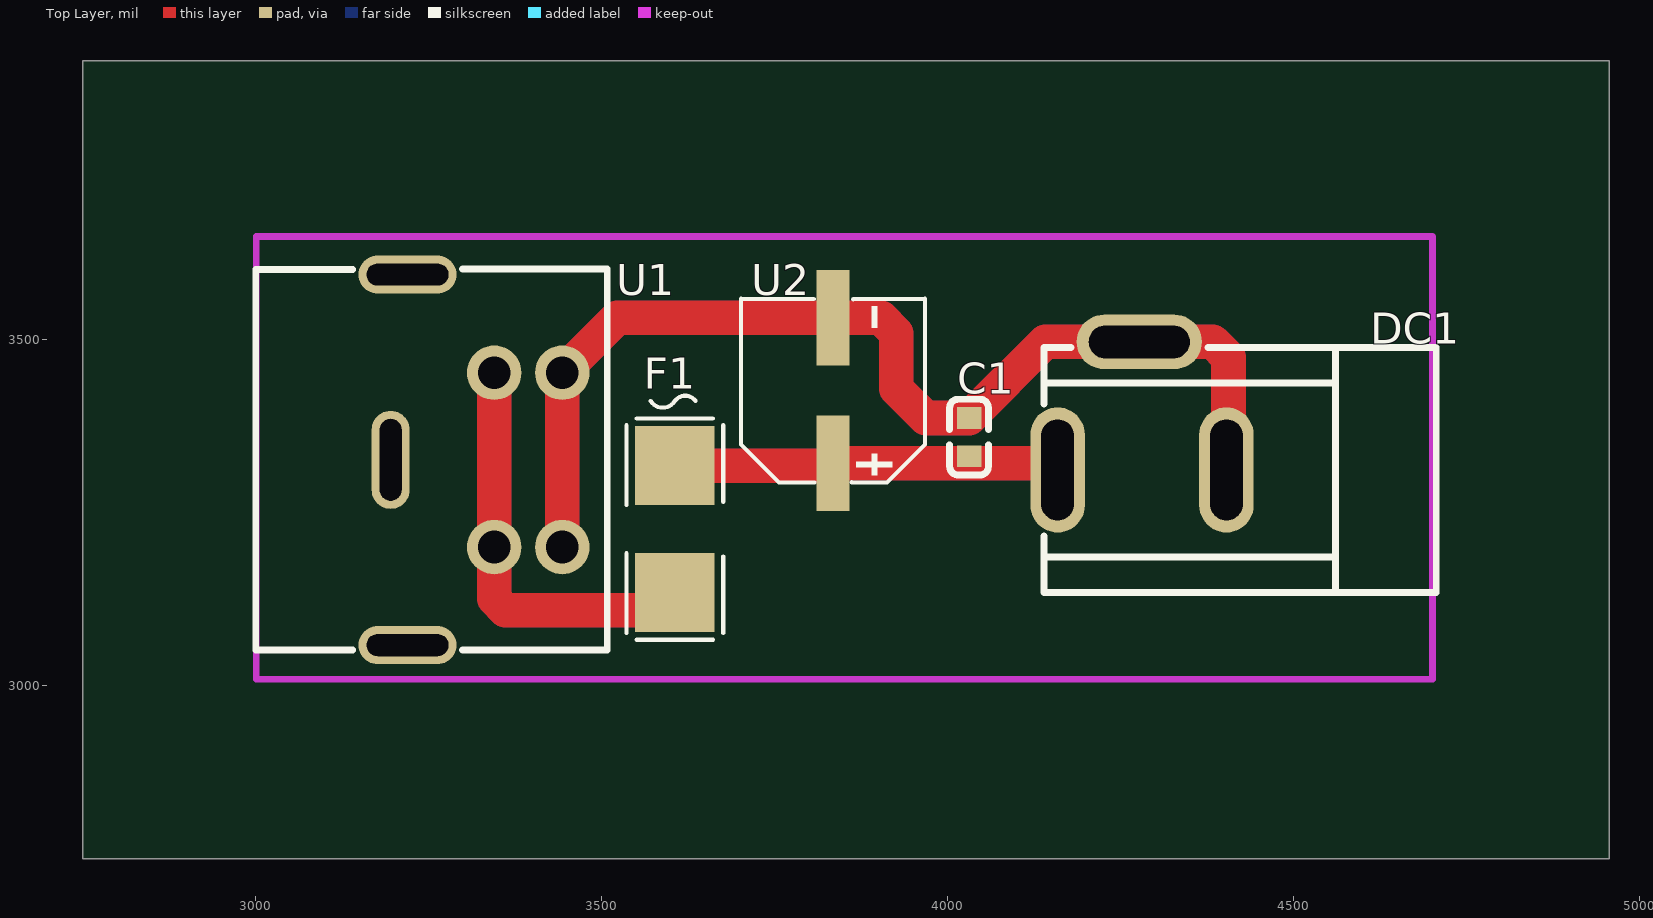
[diagram p0: Top Layer view]
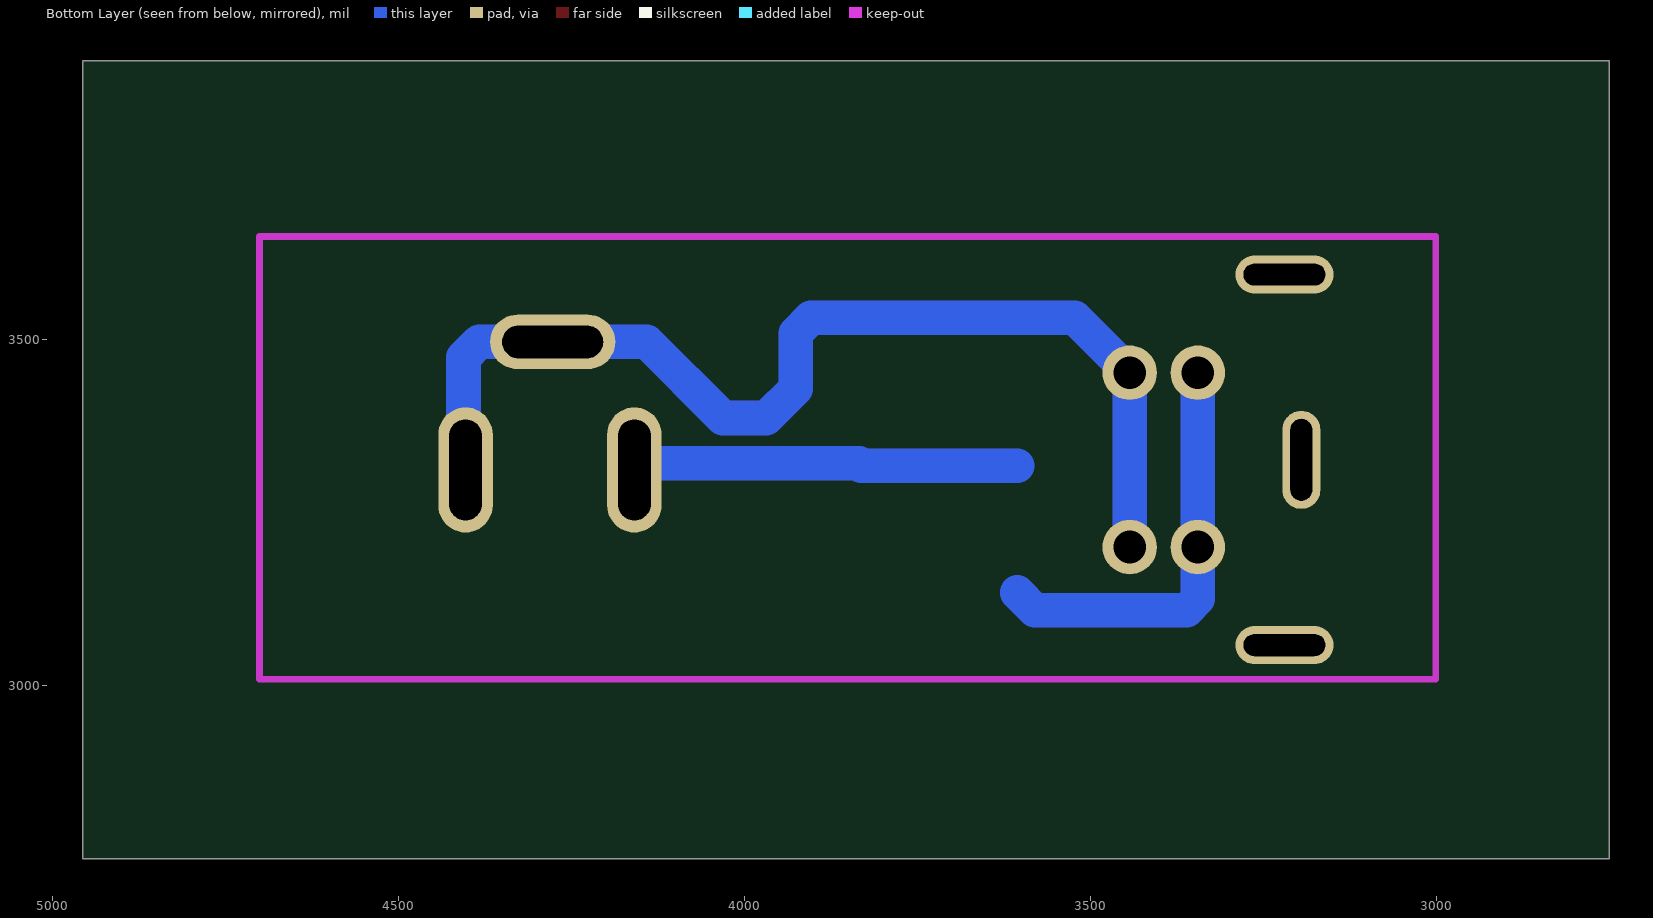
[diagram p1: Bottom Layer view, seen from below]
# Altium PCB MISC51882.pcbdoc
Units mil, origin at the board's own origin, x right, y up, seen from the top; angles counter-clockwise.
Board outline 2205.98 x 1153.54 mil, 2 copper layers (Top Layer, Bottom Layer), stack 62.206 mil thick; 5 components, 3 nets, 16 pads, 0 vias.

## Layer stack, top to bottom
Top Solder Mask Layer: solder mask 0.394, Dk 3.3
Top Layer: signal copper 1.379
Dielectric1: surface 59.449, FR4, Dk 4.5
Bottom Layer: signal copper 1.378
Bottom Solder Mask Layer: solder mask 0.394, Dk 3.3

## Board outline
4955.98,2750 2750,2750 2750,3903.54 4955.98,3903.54

## Design rules (kind name [scope] priority, off if disabled: settings)
BoardOutlineClearance copperThickness2oz_1 [All] p2 off: genericclearance=7.99 ignorepadtopadclearanceinfootprint=FALSE except(0: Arc-SplitContinuation Track-SplitContinuation SMDPad-SplitContinuation THPad-SplitContinuation Via-SplitContinuation Fill-SplitContinuation Region-SplitContinuation Poly-SplitContinuation Text-SplitContinuation Hole-SplitContinuation; 5.98: Arc-CutoutEdge SMDPad-CutoutEdge THPad-CutoutEdge Via-CutoutEdge Fill-CutoutEdge Region-CutoutEdge Text-CutoutEdge; 6.93: Hole-OutlineEdge Hole-CutoutEdge; 10: Poly-OutlineEdge Poly-CutoutEdge; 11.81: Arc-OutlineEdge Track-OutlineEdge SMDPad-OutlineEdge THPad-OutlineEdge Via-OutlineEdge Fill-OutlineEdge Region-OutlineEdge Text-OutlineEdge Track-CutoutEdge)
BoardOutlineClearance copperThickness1oz_1 [All] p4: genericclearance=4.02 ignorepadtopadclearanceinfootprint=FALSE except(0: Arc-SplitContinuation Track-SplitContinuation SMDPad-SplitContinuation THPad-SplitContinuation Via-SplitContinuation Fill-SplitContinuation Region-SplitContinuation Poly-SplitContinuation Text-SplitContinuation Hole-SplitContinuation; 6: SMDPad-CutoutEdge THPad-CutoutEdge Via-CutoutEdge Fill-CutoutEdge Region-CutoutEdge Text-CutoutEdge; 6.93: Hole-OutlineEdge Hole-CutoutEdge; 10: Poly-OutlineEdge Poly-CutoutEdge; 11.8: Arc-OutlineEdge Track-OutlineEdge SMDPad-OutlineEdge THPad-OutlineEdge Via-OutlineEdge Fill-OutlineEdge Region-OutlineEdge Text-OutlineEdge; 11.81: Arc-CutoutEdge Track-CutoutEdge)
Clearance copperThickness2oz [All] p1 off: gap=7.99 ignorepadtopadclearanceinfootprint=FALSE except(5.98: SMDPad-Track SMDPad-SMDPad THPad-Track SMDPad-THPad THPad-THPad Track-Via SMDPad-Via THPad-Via Via-Via Fill-Track Region-Track Fill-SMDPad Region-SMDPad Fill-THPad Region-THPad Fill-Via Region-Via Fill-Fill Fill-Region Region-Region Arc-Track Arc-SMDPad Arc-THPad Arc-Via Fill-Arc Region-Arc Arc-Arc Text-Track SMDPad-Text Text-THPad Text-Via Fill-Text Region-Text Arc-Text Text-Text; 6.93: Hole-Track Hole-SMDPad Hole-THPad Hole-Via Fill-Hole Region-Hole Hole-Arc Hole-Text; 10: Poly-Track Poly-SMDPad Poly-THPad Poly-Via Poly-Fill Poly-Region Poly-Poly Poly-Arc Poly-Text Poly-Hole)
Clearance copperThickness1oz [All] p3: gap=4.02 ignorepadtopadclearanceinfootprint=FALSE except(5.98: SMDPad-Track SMDPad-SMDPad THPad-Track SMDPad-THPad THPad-THPad Track-Via SMDPad-Via THPad-Via Via-Via Fill-Track Region-Track Fill-SMDPad Region-SMDPad Fill-THPad Region-THPad Fill-Via Region-Via Fill-Fill Fill-Region Region-Region; 6: Arc-Track Arc-SMDPad Arc-THPad Arc-Via Fill-Arc Region-Arc Arc-Arc Text-Track SMDPad-Text Text-THPad Text-Via Fill-Text Region-Text Arc-Text Text-Text; 6.93: Hole-Track Hole-SMDPad Hole-THPad Hole-Via Fill-Hole Region-Hole Hole-Arc Hole-Text; 10: Poly-Track Poly-SMDPad Poly-THPad Poly-Via Poly-Fill Poly-Region Poly-Poly Poly-Arc Poly-Text Poly-Hole)
DiffPairsRouting differentialPair [All] p1: maxlimit=6 minlimit=6 mostfreqgap=6 toplayer_minwidth=5 toplayer_prefwidth=10 toplayer_maxwidth=100 toplayer_mingap=6 toplayer_prefgap=6 toplayer_maxgap=6 bottomlayer_minwidth=5 bottomlayer_prefwidth=10 bottomlayer_maxwidth=100 bottomlayer_mingap=6 bottomlayer_prefgap=6 bottomlayer_maxgap=6 maxuncoupledlength=10
HoleToHoleClearance otherClearance [All] p1: gap=11.81 allowstackedmicrovias=TRUE
Length netLength [All] p1: minlimit=0 maxlimit=0
MatchedLengths netLengthTolerance [All] p1: tolerance=1000
PasteMaskExpansion pasteMaskExpansion [All] p1: expansion=0
PlaneConnect innerPlane [All] p1: planeconnectstyle=Relief reliefexpansion=20 reliefentries=4 reliefconductorwidth=10 reliefairgap=10
PolygonConnect copperRegion [All] p1: connectstyle=Relief reliefconductorwidth=10 reliefentries=4 polygonreliefangle="90 Angle" airgapwidth=10 via.connectstyle=Relief via.reliefconductorwidth=10 via.reliefentries=4 via.polygonreliefangle="90 Angle" via.airgapwidth=10
RoutingVias viaSize [All] p1: holewidth=12.01 width=24.02 viastyle="Through Hole" minholewidth=11.81 minwidth=19.68 maxholewidth=248.03 maxwidth=393.7
SolderMaskExpansion solderMaskExpansion [IsVia] p1: expansion=-1000 istentingtop=TRUE
SolderMaskExpansion solderMaskExpansion [All] p2: expansion=2 istentingtop=FALSE
Width copperThickness2oz_2 [All] p1 off: maxlimit=100 minlimit=8 preferedwidth=10
Width copperThickness1oz_2 [All] p2: maxlimit=100 minlimit=5 preferedwidth=10

## Components (designator, comment, footprint, x,y, rotation, side; value= is the part's Value field where it differs from the comment)
C1 "10uF" C0603 4030.79,3359.68 r90 top
DC1 "DC005" DC-IN-TH_DC005 4280.79,3404.68 r180 top
F1 "10A保险丝" FUSE-SMD_L6.1-W2.6 3605.67,3226.77 r270 top
U1 "M-DIN_4-R母座" CONN-TH_DIN_4P_12D8 3319.01,3326.77 r90 top
U2 "100uF贴片电解" CAP-SMD_BD6.3-L6.6-W6.6-LS7.4-FD 3834.27,3426.77 r90 top

## Footprints (in the part's own frame and the unit in brackets; to place one, negate y for a bottom-side part, rotate by r counter-clockwise, add the part's x,y. Pads: shape width x height; smd on the part's side, far side on the other; paste and mask are expansions set on the pad)
C0603 [mm]
  rect 0.8x0.9 smd: 1(-0.7,0) 2(0.7,0)
  silkscreen extent -1.39,-0.71 1.39,0.71
CAP-SMD_BD6.3-L6.6-W6.6-LS7.4-FD [mm]
  rect 3.5x1.2 smd: 1(-2.67,0) 2(2.67,0)
  silkscreen extent -3.38,-3.38 3.38,3.38
CONN-TH_DIN_4P_12D8 [mm]
  round 2 hole 1.2 paste+0 mask+0.05: 1(-3.2,-0.65) 2(3.2,-0.65) 3(3.2,-3.15) 4(-3.2,-3.15)
  oval 3.6x1.4 hole 0.8 slot 3 at 0 deg paste+0 mask+0.05: 5(0,3.15)
  oval 1.4x3.6 hole 0.8 slot 3 at 90 deg paste+0 mask+0.05: 6(-6.8,2.53) 7(6.8,2.53)
  silkscreen extent -6.98,-4.8 7,8.1
DC-IN-TH_DC005 [mm]
  oval 2x4.6 hole 1.2 slot 3.7 at 90 deg: 1(3.1,2.35) 2(-3.1,2.35)
  oval 4.6x2 hole 1.2 slot 3.7 at 0 deg: 3(0.1,-2.35)
  silkscreen extent -10.8,-2.15 3.6,6.85
FUSE-SMD_L6.1-W2.6 [mm]
  rect 2.91x2.911 smd paste-100 mask+0.051: 1(-2.33,0) 2(2.33,0)
  silkscreen extent -4.89,-1.78 4.06,1.78

## Nets (pads, with @x,y where several pads share a name; then routed paths per layer and width w, separated by ;. In a path a pad name is that pad's centre, name@x,y a point inside that pad or via, vN(x,y) a via of type N, cw(c..) or ccw(c..) an arc to the next point about the centre after c; other vN are vias at no path point)
$1N1: F1.2 U1.1 U1.2 | length 1210.3
  Top Layer w50: U1.2 U1.1 3344.6,3125.87 3360.79,3109.68 3580.31,3109.68 F1.2
  Bottom Layer w50: U1.2 U1.1 3344.6,3125.87 3360.79,3109.68 3580.31,3109.68 3605.67,3135.04
$1N2: C1.1 DC1.1 F1.1 U2.1 | length 1116.6
  Top Layer w50: F1.1 3831.12,3318.5 U2.1 4149.26,3321.66 DC1.1
  Bottom Layer w50: 3605.67,3318.5 3831.12,3318.5 3834.27,3321.66 4149.26,3321.66 DC1.1
$1N3: C1.2 DC1.2 DC1.3 U1.3 U1.4 U2.2 | length 3145.8
  Top Layer w50: U1.4 U1.3 3522.16,3531.89 U2.2 3903.59,3531.89 3925.79,3509.68 3925.79,3429.68 3968.23,3387.24 C1.2 4140.75,3497.21 DC1.3 4383.26,3497.21 4405.79,3474.68 4405.79,3315.12 DC1.2
  Bottom Layer w50: U1.4 U1.3 3522.16,3531.89 3903.59,3531.89 3925.79,3509.68 3925.79,3429.68 3968.23,3387.24 4030.79,3387.24 4140.75,3497.21 DC1.3 4383.26,3497.21 4405.79,3474.68 4405.79,3315.12 DC1.2
pads on no net: U1.5 U1.6 U1.7

## Keep-outs
Board Outline Layer:
  lines w10: 3000.79,3009.68 3000.79,3649.68 4700.79,3649.68 4700.79,3009.68 3000.79,3009.68